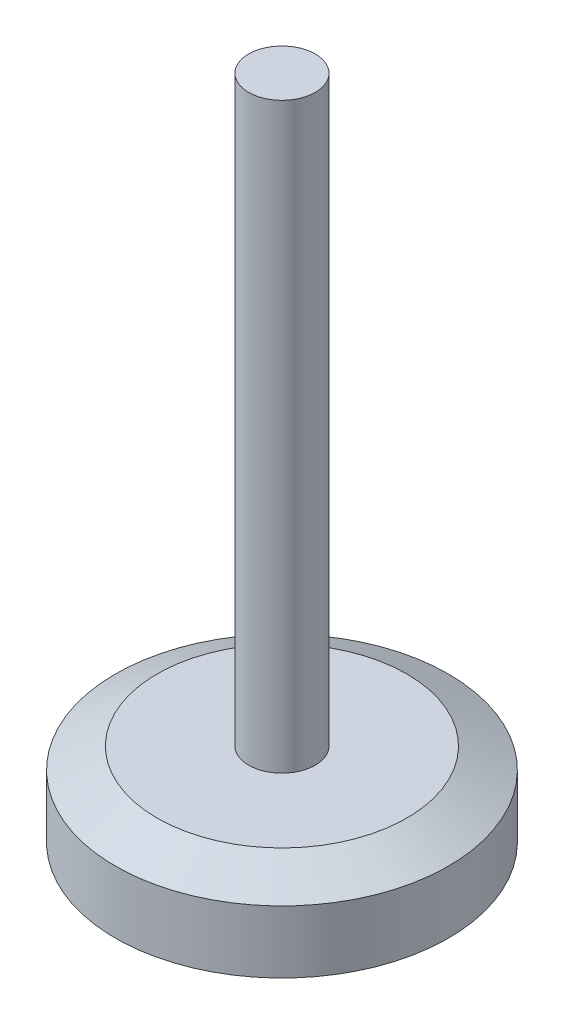
SolidWorks part; units mm, degrees
ref_plane "前视基准面" through (0, 0, 0) normal (0, 0, 1) x (1, 0, 0)
ref_plane "上视基准面" through (0, 0, 0) normal (0, 1, 0) x (1, 0, 0)
ref_plane "右视基准面" through (0, 0, 0) normal (1, 0, 0) x (0, 0, -1)
sketch "草图1" plane through (0, 0, 0) normal (0, 0, 1) x (1, 0, 0)
  line L0 (0, 0) -> (0, 116.4587) construction
  line L1 (0, 0) -> (40, 0)
  line L2 (40, 0) -> (40, 15)
  line L3 (40, 15) -> (30, 20)
  line L4 (30, 20) -> (8, 20)
  line L5 (8, 20) -> (8, 160)
  line L6 (8, 160) -> (0, 160)
  line L7 (0, 160) -> (0, 0)
  dimension "D1" = 8
  dimension "D2" = 40
  dimension "D3" = 15
  dimension "D4" = 20
  dimension "D5" = 30
  dimension "D6" = 160
revolve "旋转1" add sketch "草图1" angle 360 about L0
cosmetic thread "装饰螺纹线1"
